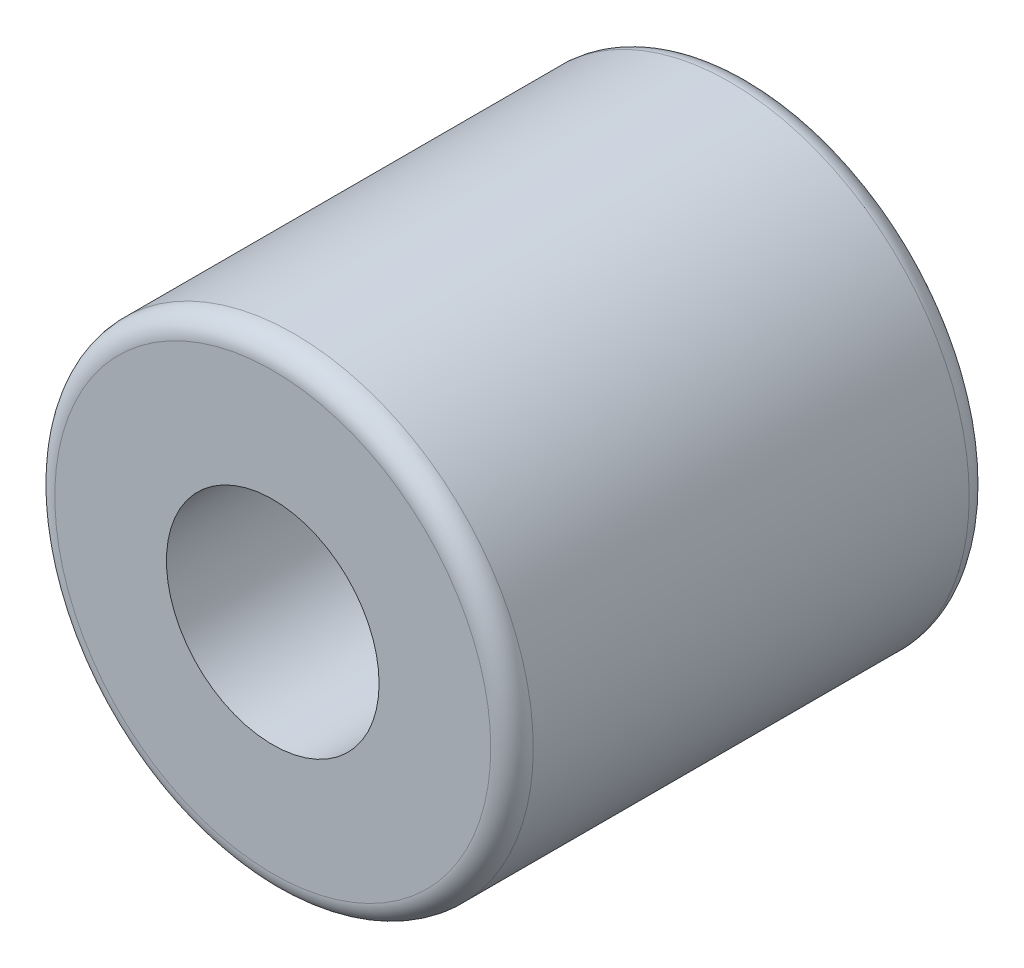
SolidWorks part; units mm, degrees
ref_plane "前视基准面" through (0, 0, 0) normal (0, 0, 1) x (1, 0, 0)
ref_plane "上视基准面" through (0, 0, 0) normal (0, 1, 0) x (1, 0, 0)
ref_plane "右视基准面" through (0, 0, 0) normal (1, 0, 0) x (0, 0, -1)
sketch "草图1" plane through (0, 0, 0) normal (0, 0, 1) x (1, 0, 0)
  circle A0 centre (0, 0) radius 22.5
  dimension "D1" = 45
extrude "凸台-拉伸1" add sketch "草图1" along normal blind 45
fillet "圆角1" radius 2 2 edges at (22.5, 0, 45) (22.5, 0, 0)
sketch "草图2" plane through (0, 0, 45) normal (0, 0, 1) x (1, 0, 0)
  circle A0 centre (0, 0) radius 10
  dimension "D1" = 20
extrude "切除-拉伸1" cut sketch "草图2" against normal through all
